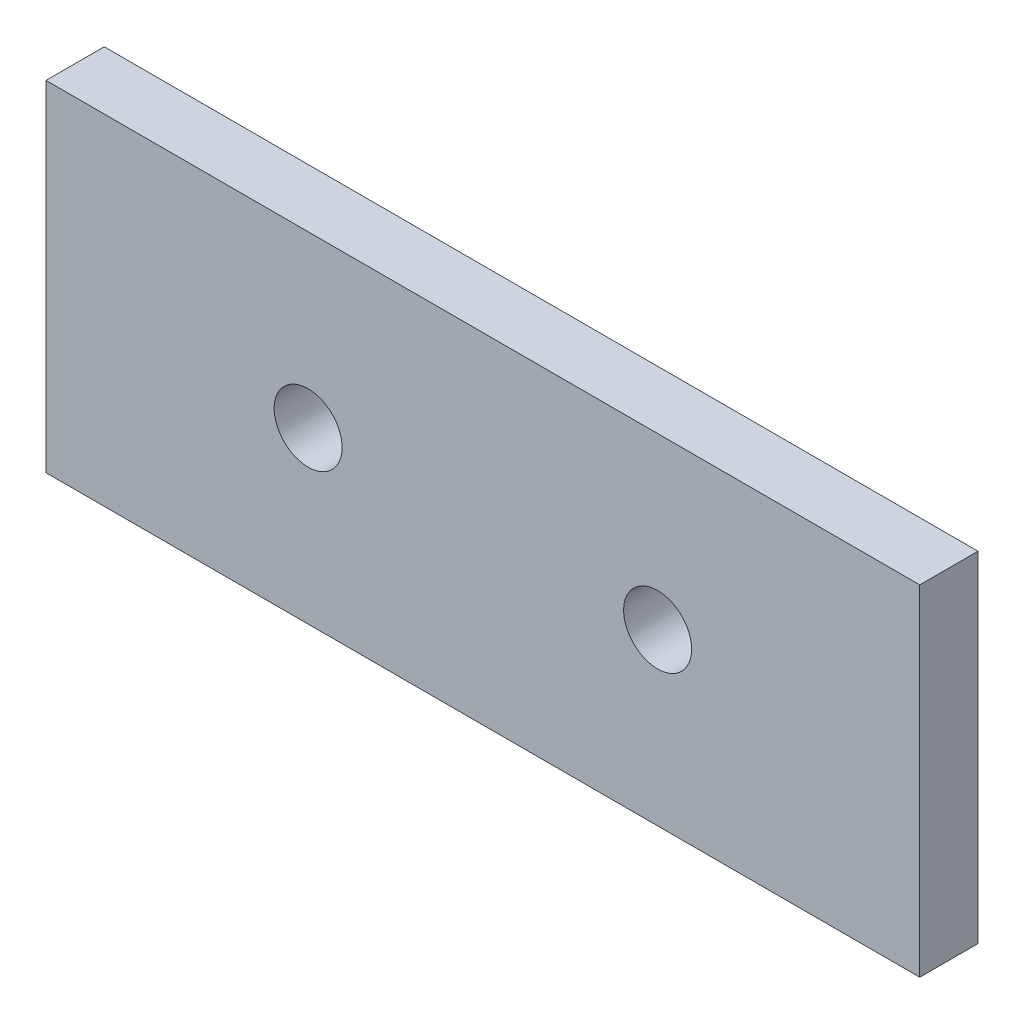
SolidWorks part; units mm, degrees
material "Q235"
ref_plane "Front Plane" through (0, 0, 0) normal (0, 0, 1) x (1, 0, 0)
ref_plane "Top Plane" through (0, 0, 0) normal (0, 1, 0) x (1, 0, 0)
ref_plane "Right Plane" through (0, 0, 0) normal (1, 0, 0) x (0, 0, -1)
sketch "Sketch1" plane through (0, 0, 0) normal (0, 0, 1) x (1, 0, 0)
  line L1 (0, 0) -> (90, 0)
  line L2 (0, 0) -> (0, 35)
  line L3 (0, 35) -> (90, 35)
  line L4 (90, 0) -> (90, 35)
  dimension "D1" = 35
  dimension "D2" = 90
extrude "Boss-Extrude1" add sketch "Sketch1" along normal blind 6
hole_wizard "M6 Clearance Hole1" positions "Sketch2" profile "Sketch3" hole size "M6" standard "GB" end condition through all
sketch "Sketch2" plane through (0, 0, 6) normal (0, 0, 1) x (1, 0, 0)
  line L0 (45, 35) -> (45, 0) construction
  line L1 (90, 35) -> (0, 35) construction
  line L2 (0, 0) -> (90, 0) construction
  point P0 (27, 17.5)
  point P2 (63, 17.5)
  dimension "D1" = 36
  dimension "D2" = 17.5
sketch "Sketch3" plane through (27, 17.5, 6) normal (1, 0, 0) x (0, -1, 0)
  line L0 (0, 0) -> (0, 6)
  line L1 (0, 6) -> (3.5, 6)
  line L2 (3.5, 6) -> (3.5, 0)
  line L5 (3.5, 0) -> (0, 0)
  line L11 (0, -6.35) -> (0, 107.95) construction
  dimension "通孔孔直径" = 7
  dimension "通孔孔深度" = 6
